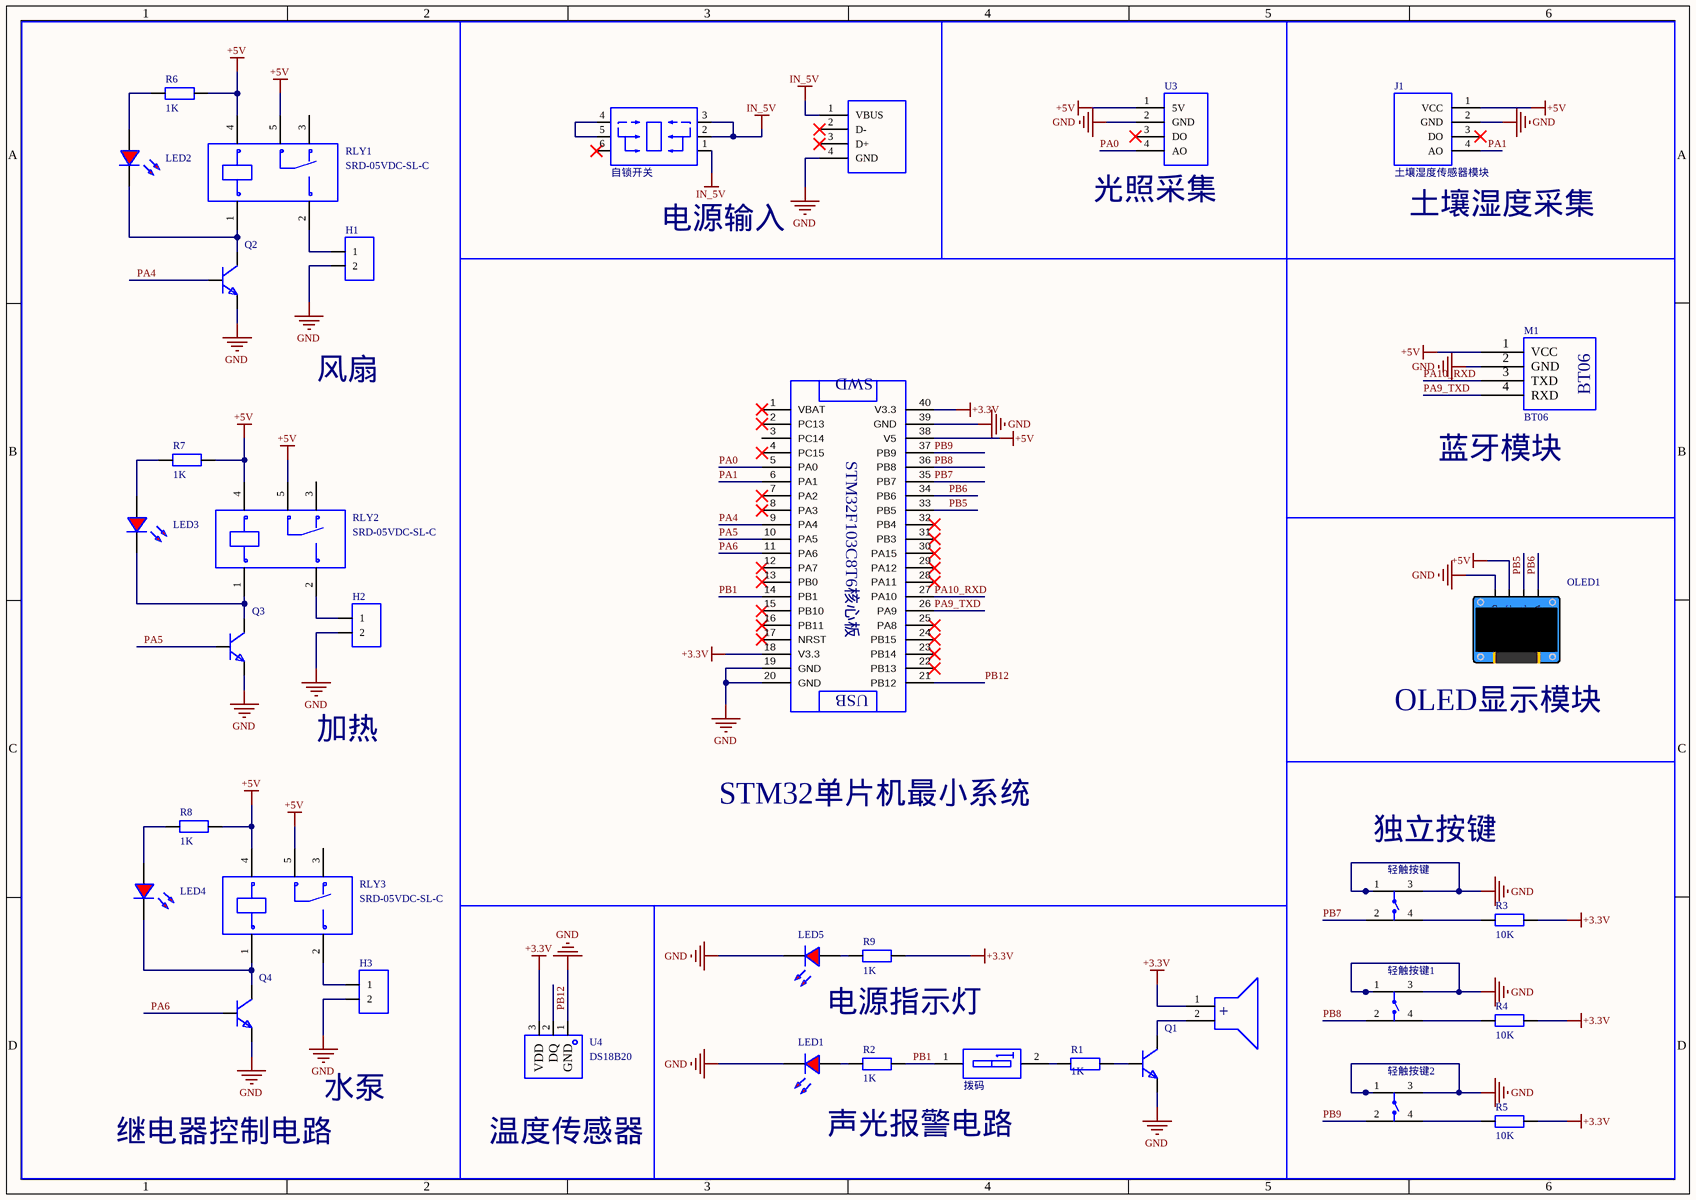
[diagram p0: MISC51322-3.schdoc]
# Altium project MISC51322-2.PrjPcb
1 sheet, 37 parts. Net scope: global (net labels, ports and power ports of the same name join across sheets).
Board file: MISC51322.pcbdoc

## Sheet MISC51322-3.schdoc
size 297 x 209 mm; Version: V1.0; @Project Name: MISC51322; @Update Date: 2026-04-15; @Create Date: 2026-04-15; @Board Name: MISC51322; @Create Time: 20:17:51; @Page Count: 1; @Page No: 1; @Schematic Name: MISC51322; @Update Time: 20:17:51; Size: A4

### Parts
BUZZER1  3kHz  [BUZ-TH_BD9.0-P5.00-D0.6-FD]  (value not drawn)
H1  (no value)  [HDR-TH_2P-P2.54-V-F]
H2  (no value)  [HDR-TH_2P-P2.54-V-F]
H3  (no value)  [HDR-TH_2P-P2.54-V-F]
J1  土壤湿度传感器模块  [Hearder-4]
LED1  (no value)  [LED-TH_5mm]
LED2  (no value)  [LED-TH_5mm]
LED3  (no value)  [LED-TH_5mm]
LED4  (no value)  [LED-TH_5mm]
LED5  (no value)  [LED-TH_5mm]
M1  BT06  [BT06]
OLED1  (no value)  [0.96OLED_4P]
Q1  S8050  [SOT-23-3_L2.9-W1.3-P1.90-LS2.3-BR]  (value not drawn)
Q2  S8050  [SOT-23-3_L2.9-W1.3-P1.90-LS2.3-BR]  (value not drawn)
Q3  S8050  [SOT-23-3_L2.9-W1.3-P1.90-LS2.3-BR]  (value not drawn)
Q4  S8050  [SOT-23-3_L2.9-W1.3-P1.90-LS2.3-BR]  (value not drawn)
R1  1K  [R0805]
R2  1K  [R0805]
R3  10K  [R0805]
R4  10K  [R0805]
R5  10K  [R0805]
R6  1K  [R0805]
R7  1K  [R0805]
R8  1K  [R0805]
R9  1K  [R0805]
RLY1  SRD-05VDC-SL-C  [RELAY-TH_SRD-XXVDC-XL-C]
RLY2  SRD-05VDC-SL-C  [RELAY-TH_SRD-XXVDC-XL-C]
RLY3  SRD-05VDC-SL-C  [RELAY-TH_SRD-XXVDC-XL-C]
SW1  自锁开关  [SW-TH_6P-L8.5-W8.5-P2.50-LS5.5-BL-2]
SW2  拨码  [SW-TH_DSWB01LHGET]
U1  (no value)  [USB-type-C模块]
U2  CW32F030C8最小系统板  [STM32F103C8T6核心板]  (value not drawn)
U3  (no value)  [光敏传感器模块]
U4  DS18B20  [3p_2.54]
轻触按键  SH-6X6X6.5H-TP  [SW-SMD_4P-L6.2-W6.2-P4.50-LS9.5-TL]  (value not drawn)
轻触按键1  SH-6X6X6.5H-TP  [SW-SMD_4P-L6.0-W6.0-P4.50-LS8.8]  (value not drawn)
轻触按键2  SH-6X6X6.5H-TP  [SW-SMD_4P-L6.0-W6.0-P4.50-LS8.8]  (value not drawn)

### Blocks framed on the sheet
电源输入: SW1 U1
光照采集: U3
土壤湿度采集: J1
蓝牙模块: M1
OLED显示模块: OLED1
独立按键: R3-R5 轻触按键 轻触按键1 轻触按键2
温度传感器: U4

### Nets
+3.3V: BUZZER1.1(+) R3.2 R4.2 R5.2 R9.2 U2.18(V3.3) U2.40(V3.3) U4.3(VDD)
+5V: J1.1(VCC) M1.1(VCC) OLED1.2(VCC) R6.1 R7.1 R8.1 RLY1.4 RLY1.5 RLY2.4 RLY2.5 RLY3.4 RLY3.5 U2.38(V5) U3.1(5V)
GND: H1.2 H2.2 H3.2 J1.2(GND) LED1.2(A) LED5.2(A) M1.2(GND) OLED1.1(GND) Q1.2(E) Q2.2(E) Q3.2(E) Q4.2(E) U1.4(GND) U2.19(GND) U2.20(GND) U2.39(GND) U3.2(GND) U4.1(GND) 轻触按键.1 轻触按键.3 轻触按键1.1 轻触按键1.3 轻触按键2.1 轻触按键2.3
IN_5V: SW1.1 SW1.2 SW1.3 U1.1(VBUS)
PA0: U2.5(PA0) U3.4(AO)
PA1: J1.4(AO) U2.6(PA1)
PA4: Q2.1(B) U2.9(PA4)
PA5: Q3.1(B) U2.10(PA5)
PA6: Q4.1(B) U2.11(PA6)
PA9_TXD: M1.4(RXD) U2.26(PA9)
PA10_RXD: M1.3(TXD) U2.27(PA10)
PB1: R2.2 SW2.1(A1) U2.14(PB1)
PB5: OLED1.3(SCL) U2.33(PB5)
PB6: OLED1.4(SDA) U2.34(PB6)
PB7: U2.35(PB7) 轻触按键.2
PB8: U2.36(PB8) 轻触按键1.2
PB9: U2.37(PB9) 轻触按键2.2
PB12: U2.21(PB12) U4.2(DQ)
NetBUZZER1_2: BUZZER1.2(-) Q1.3(C)
NetH1_1: H1.1 RLY1.2
NetH2_1: H2.1 RLY2.2
NetH3_1: H3.1 RLY3.2
NetLED1_1: LED1.1(C) R2.1
NetLED2_1: LED2.1(C) R6.2
NetLED2_2: LED2.2(A) Q2.3(C) RLY1.1
NetLED3_1: LED3.1(C) R7.2
NetLED3_2: LED3.2(A) Q3.3(C) RLY2.1
NetLED4_1: LED4.1(C) R8.2
NetLED4_2: LED4.2(A) Q4.3(C) RLY3.1
NetLED5_1: LED5.1(C) R9.1
NetQ1_1: Q1.1(B) R1.2
NetR1_1: R1.1 SW2.2
NetR3_1: R3.1 轻触按键.4
NetR4_1: R4.1 轻触按键1.4
NetR5_1: R5.1 轻触按键2.4
NetSW1_4: SW1.4 SW1.5

Not connected (* = marked no-connect by the designer): J1 3(DO)*; RLY1 3; RLY2 3; RLY3 3; SW1 6*; U1 2(D-)* 3(D+)*; U2 1(VBAT)* 2(PC13)* 3(PC14) 4(PC15)* 7(PA2)* 8(PA3)* 12(PA7)* 13(PB0)* 15(PB10)* 16(PB11)* 17(NRST)* 22(PB13)* 23(PB14)* 24(PB15)* 25(PA8)* 28(PA11)* 29(PA12)* 30(PA15)* 31(PB3)* 32(PB4)*; U3 3(DO)*

### Notes on the sheet
- 风扇
- 加热
- STM32单片机最小系统
- 电源指示灯
- 继电器控制电路
- 水泵
- 声光报警电路

### Library data of the parts
BUZZER1 = HNB09A03: 驱动方式:有源(内含驱动线路);构造类型:电磁式;频率:3kHz;声压(SPL):85dB;; Manufacturer: 华能; AddInBom: yes; ModelId: 13273335caac486e928bafb4d9fdf12d0819f05c4eef4c71ace90d822a990e87; ModelName: BUZ-TH_D9.0-H5.5-P5.0; ModelTransform: 354.33,354.33,0,90,0,0,-0.005,0,-177.165; Voltage - Supply: 1.5V~4.5V; Current Consumption: 30mA; Sound Pressure Level(SPL): 85dB; Symbol: HNB09A03; Device: HNB09A03; LCSC Part Name: 电磁式有源一体蜂鸣器HNB09A03; SupplierPart: C96102; ManufacturerPart: HNB09A03; Supplier Footprint: 插件,D=9mm; JLCPCB Part Class: Extended Part; Datasheet: https://item.szlcsc.com/datasheet/HNB09A03/97306.html; Supplier: LCSC; ConvertToPcb: yes; FootprintName: BUZ-TH_BD9.0-P5.00-D0.6-FD; Driver Circuitry: 有源(内含驱动线路); Technology: 电磁式; Value: 3kHz; Diameter(φD): 9mm; Length: -; Width: -; Height: 5.5mm; Operating Temperature: -20℃~+70℃
H1-H3 = HDR-F_2.54_1x2P: Symbol: Header-Female-2.54_1x2; ConvertToPcb: yes; ModelId: a9450ef445564560a104363b9aacde4e0819f05c4eef4c71ace90d822a990e87; ModelName: HDR-TH_2P-P2.54-F-LI-1X2P; ModelTransform: 215.7476,98.425,0,0,0,0,0,0,-129.921; Device: HDR-F_2.54_1x2P; AddInBom: yes; SupplierPart: C49661; Supplier Footprint: 插件; FootprintName: HDR-TH_2P-P2.54-V-F
J1 = 土壤湿度传感器模块: AddInBom: yes; Symbol: 土壤湿度传感器模块; Device: 土壤湿度传感器模块; ConvertToPcb: yes; FootprintName: Hearder-4
LED1 = LED_TH-R_5mm: ConvertToPcb: yes; ModelId: fe9cea1bdf7642cd8d9a5077ed0e2b580819f05c4eef4c71ace90d822a990e87; ModelName: LED-TH_BD5.9-P2.54-RD_RED; ModelTransform: 222.16,238.98,581.81,180,0,0,-6,0,-220; Symbol: LED_TH-R; Device: LED_TH-R_5mm; AddInBom: yes; FootprintName: LED-TH_5mm; Supplier Footprint: 插件
LED2-LED5 = LED_TH-R_5mm: 3D Model: fe9cea1bdf7642cd8d9a5077ed0e2b580819f05c4eef4c71ace90d822a990e87; 3D Model Transform: 222.16,238.98,581.81,180,0,0,-6,0,-220; ConvertToPcb: yes; ModelName: LED-TH_BD5.9-P2.54-RD_RED; Symbol: LED_TH-R; Device: LED_TH-R_5mm; Supplier Footprint: 插件; AddInBom: yes; FootprintName: LED-TH_5mm
M1 = BT06: AddInBom: yes; Symbol: BT06; Device: BT06; ConvertToPcb: yes
OLED1 = 0.96OLED模块_4P: ConvertToPcb: yes; ModelId: 79c000fdb68d45a296c2e9bedf4f90550819f05c4eef4c71ace90d822a990e87; ModelTransform: 1393.69792,1318.895,0,0,0,0,0,-560.079,-137.795; Symbol: 0.96OLED模块_4P; Device: 0.96OLED模块_4P; AddInBom: yes; FootprintName: 0.96OLED_4P; Supplier Footprint: 插件; ModelName: 0.96OLED_4P
Q1 = S8050_C20069125: 晶体管类型:NPN;集电极电流(Ic):500mA;集射极击穿电压(Vceo):25V;耗散功率(Pd):300mW;直流电流增益(hFE):120@50mA,1.0V;; Manufacturer: R+O(宏嘉诚); AddInBom: yes; ModelId: 5504beb8757f4de79731898ec55d3e540819f05c4eef4c71ace90d822a990e87; ModelTransform: 114.173,90.551,0,90,0,0,0,0,0; type: NPN; Current - Collector(Ic): 500mA; Collector - Emitter Voltage VCEO: 25V; Pd - Power Dissipation: 300mW; Transition frequency(fT): 100MHz; Current - Collector Cutoff: 100nA; Vce Saturation(VCE(sat)): 600mV@500mA,50mA; Emitter-Base Voltage(Vebo): 5V; Symbol: S8050_C20069125; Device: S8050_C20069125; LCSC Part Name: hFE:200-350，丝印:J3Y NPN 500mA 25V; SupplierPart: C20069125; ManufacturerPart: S8050; Supplier Footprint: SOT-23; JLCPCB Part Class: Extended Part; Datasheet: https://item.szlcsc.com/datasheet/S8050/21397163.html; Supplier: LCSC; ConvertToPcb: yes; FootprintName: SOT-23-3_L2.9-W1.3-P1.90-LS2.3-BR; ModelName: SOT-23-3_L2.9-W1.3-P1.90-LS2.3-BR; DC Current Gain: 120@50mA,1.0V; Operating Temperature: -55℃~+150℃
Q2-Q4 = S8050_C20069125: 晶体管类型:NPN;集电极电流(Ic):500mA;集射极击穿电压(Vceo):25V;耗散功率(Pd):300mW;直流电流增益(hFE):120@50mA,1.0V;; Manufacturer: R+O(宏嘉诚); 3D Model: 5504beb8757f4de79731898ec55d3e540819f05c4eef4c71ace90d822a990e87; 3D Model Transform: 114.173,90.551,0,90,0,0,0,0,0; type: NPN; Current - Collector(Ic): 500mA; Collector - Emitter Voltage VCEO: 25V; Pd - Power Dissipation: 300mW; Transition frequency(fT): 100MHz; Current - Collector Cutoff: 100nA; Vce Saturation(VCE(sat)): 600mV@500mA,50mA; Emitter-Base Voltage(Vebo): 5V; AddInBom: yes; Symbol: S8050_C20069125; Device: S8050_C20069125; LCSC Part Name: hFE:200-350，丝印:J3Y NPN 500mA 25V; Supplier Part: C20069125; Manufacturer Part: S8050; Supplier Footprint: SOT-23; JLCPCB Part Class: Extended Part; Datasheet: https://item.szlcsc.com/datasheet/S8050/21397163.html; Supplier: LCSC; DC Current Gain: 120@50mA,1.0V; Operating Temperature: -55℃~+150℃; ConvertToPcb: yes; FootprintName: SOT-23-3_L2.9-W1.3-P1.90-LS2.3-BR; ModelName: SOT-23-3_L2.9-W1.3-P1.90-LS2.3-BR
R1 R2 = Res_0805: Symbol: 电阻; ConvertToPcb: yes; ModelId: 37a81e68749a4138bd2dfa6897b24b850819f05c4eef4c71ace90d822a990e87; ModelName: R0805_L2.0-W1.3-H0.6; ModelTransform: 78.74,51.181,0,0,0,0,0,-0.0005,0; Device: Res_0805; Value: 1K; AddInBom: yes; Supplier Footprint: 0805; FootprintName: R0805
R3-R9 = Res_0805: Symbol: 电阻; 3D Model: 37a81e68749a4138bd2dfa6897b24b850819f05c4eef4c71ace90d822a990e87; 3D Model Transform: 78.74,51.181,0,0,0,0,0,-0.0005,0; ConvertToPcb: yes; ModelName: R0805_L2.0-W1.3-H0.6; Device: Res_0805; Supplier Footprint: 0805; AddInBom: yes; FootprintName: R0805
  R3-R5: Value: 10K
  R6-R9: Value: 1K
RLY1-RLY3 = SRD-05VDC-SL-C: 线圈电压:5V;触点形式:一组转换:1C(单刀双掷-转换);触点容量(电阻负载):-;最大切换电压:250V@AC;最大切换电流:15A;; Manufacturer: 松乐; AddInBom: yes; ModelId: d0eda9b8bf8746d18ae810ab88dc78e70819f05c4eef4c71ace90d822a990e87; ModelName: RELAY-TH_L19.2-W15.6-H15.8; ModelTransform: 755.904,622.4397,0,0,0,0,34.882,0,-118.11; Coil Voltage: 5V; Coil Rated Power: 360mW; Switching Current(Max): 15A; Coil Type: 无极性-单线圈; Coil Resistance: 70Ω; Contact Resistance: 100mΩ; Operate Time: 10ms; Symbol: SRD-05VDC-SL-C; Device: SRD-05VDC-SL-C; LCSC Part Name: 蓝色 单组转换型继电器; SupplierPart: C35449; ManufacturerPart: SRD-05VDC-SL-C; Supplier Footprint: 插件,15.6x19.2mm; JLCPCB Part Class: Extended Part; Datasheet: https://item.szlcsc.com/datasheet/SRD-05VDC-SL-C/36422.html; Supplier: LCSC; ConvertToPcb: yes; FootprintName: RELAY-TH_SRD-XXVDC-XL-C; Contact Form: 一组转换:1C(单刀双掷-转换); Number of Pins: 5; Contact Rating: -; Switching Voltage(Max): 250V@AC; Release Time: 10ms
SW1 = PS851-06L140E1-ZCY-G: 8.5x8.5x14，6只端子、自锁、底座黑色、盖板灰色; Manufacturer: Khon(康宏电子); AddInBom: yes; ModelId: 3d3c155482f1468c89deb1ae1eab44490819f05c4eef4c71ace90d822a990e87; ModelTransform: 334.645,335.0387,0,0,0,0,0,0,-137.795; Symbol: PS851-06L140E1-ZCY-G; Device: PS851-06L140E1-ZCY-G; Manufacturer Part: 自锁开关; LCSC Part Name: 8.5x8.5自锁开关; SupplierPart: C46533678; Supplier Footprint: DIP-6P,8.5x8.5mm; Datasheet: https://item.szlcsc.com/datasheet/PS851-06L140E1-ZCY-G/48661192.html; Supplier: LCSC; ConvertToPcb: yes; FootprintName: SW-TH_6P-L8.5-W8.5-P2.50-LS5.5-BL-2; ModelName: SW-TH_6P-L8.5-W8.5-P2.50-LS5.5-BL-2
SW2 = DSWB01LHGET: 类型:平拨,凸起式;电路结构:单刀单掷;开关位数:1位;工作寿命:-;颜色:红色;; Manufacturer: YE; AddInBom: yes; ModelId: 0f47cc4368c24d779ddaf17d8f9a8b630819f05c4eef4c71ace90d822a990e87; ModelName: SW-TH_2P-L4.1-W9.9-H5.4-P2.54; ModelTransform: 161.417,389.763,0,0,0,0,2.205,-1.024,-125.984; Circuit: 单刀单掷; Number of Positions: 1位; Symbol: DSWB01LHGET; Device: DSWB01LHGET; Manufacturer Part: 拨码; LCSC Part Name: 红色宽体1位顶拨插件; SupplierPart: C126888; Supplier Footprint: 插件,9.9x4mm; JLCPCB Part Class: Extended Part; Datasheet: https://item.szlcsc.com/datasheet/DSWB01LHGET/138168.html; Supplier: LCSC; ConvertToPcb: yes; FootprintName: SW-TH_DSWB01LHGET; Type: 平拨,凸起式; Lead Pitch: -; Operating Life: -; Color: 红色
U1 = TYPE-C模块: AddInBom: yes; Symbol: TYPE-C模块; Device: TYPE-C模块; ConvertToPcb: yes
U2 = STM32F103C8T6最小系统: Manufacturer: 无; ManufacturerPart: STM32F103C8T6最小系统模块; Symbol: STM32F103C8T6最小系统_1; AddInBom: yes; tags: STM32; Device: STM32F103C8T6最小系统; ConvertToPcb: yes; SupplierPart: C8734; OriginFootprint: STM32F103C8T6核心板; JLCPCB Part Class: Basic Part; FootprintName: STM32F103C8T6核心板
U3 = 光敏传感器模块: AddInBom: yes; Symbol: 光敏传感器模块; Device: 光敏传感器模块; ConvertToPcb: yes; FootprintName: 光敏传感器模块
U4 = DS18B20: Manufacturer: UMW(友台半导体); AddInBom: yes; Symbol: DS18B20; Device: DS18B20; ConvertToPcb: yes; Supplier: LCSC; SupplierPart: C376006; ManufacturerPart: DS18B20; JLCPCB Part Class: Extended Part
轻触按键 = SH-6X6X6.5H-TP: 电路结构:单刀单掷;按钮形状:圆形按钮;作用力:2.5N;安装方式:立贴;开关长度:6mm;开关宽度:6mm;开关高度:6.5mm;带支架:不带支架;触点电流:50mA;额定电压:12V;带灯:无;工作寿命:10万次;; Manufacturer: SHOU HAN(首韩); AddInBom: yes; Circuit: 单刀单掷; Actuator Style: 圆形按钮; Operating Force: 2.5N; Switch Height: 6.5mm; with Bracket: 不带支架; Contact Current: 50mA; Voltage Rating: 12V; Actuator/Cap Color: 黑色; With Lamp: 无; Life: 10万次; Symbol: SH-6X6X6.5H-TP; Device: SH-6X6X6.5H-TP; LCSC Part Name: 6*6/6x6 轻触开关; SupplierPart: C42416255; ManufacturerPart: SH-6X6X6.5H-TP; Supplier Footprint: SMD-4P,6x6mm; JLCPCB Part Class: Extended Part; Datasheet: https://item.szlcsc.com/datasheet/SH-6X6X6.5H-TP/44415302.html; Supplier: LCSC; ConvertToPcb: yes; FootprintName: SW-SMD_4P-L6.2-W6.2-P4.50-LS9.5-TL; Mounting Type: 立贴; Length: 6mm; Width: 6mm; Termination Style: 鸥翼型; Operating Temperature: -25℃~+70℃
轻触按键1 轻触按键2 = SH-6X6X6.5H-TP: 电路结构:单刀单掷;按钮形状:圆形按钮;作用力:2.5N;安装方式:立贴;开关长度:6mm;开关宽度:6mm;开关高度:6.5mm;带支架:不带支架;触点电流:50mA;额定电压:12V;带灯:无;工作寿命:10万次;; Manufacturer: SHOU HAN(首韩); Circuit: 单刀单掷; Actuator Style: 圆形按钮; Operating Force: 2.5N; Switch Height: 6.5mm; with Bracket: 不带支架; Contact Current: 50mA; Voltage Rating: 12V; Actuator/Cap Color: 黑色; With Lamp: 无; Life: 10万次; AddInBom: yes; Symbol: SH-6X6X6.5H-TP; Device: SH-6X6X6.5H-TP; LCSC Part Name: 6*6/6x6 轻触开关; Supplier Part: C42416255; Manufacturer Part: SH-6X6X6.5H-TP; Supplier Footprint: SMD-4P,6x6mm; JLCPCB Part Class: Extended Part; Datasheet: https://item.szlcsc.com/datasheet/SH-6X6X6.5H-TP/44415302.html; Supplier: LCSC; Mounting Type: 立贴; Length: 6mm; Width: 6mm; Termination Style: 鸥翼型; Operating Temperature: -25℃~+70℃; ConvertToPcb: yes; FootprintName: SW-SMD_4P-L6.0-W6.0-P4.50-LS8.8